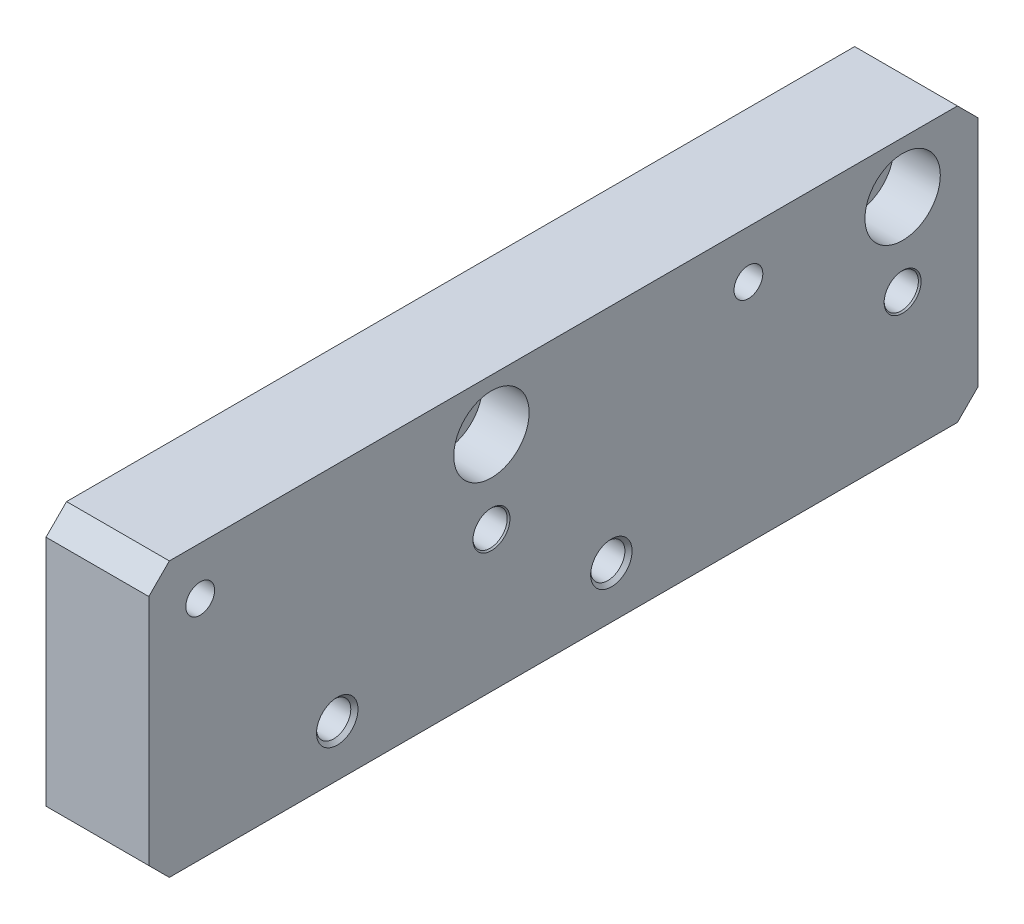
SolidWorks part; units mm, degrees
material "6061-T6"
ref_plane "Front Plane" through (0, 0, 0) normal (0, 0, 1) x (1, 0, 0)
ref_plane "Top Plane" through (0, 0, 0) normal (0, 1, 0) x (1, 0, 0)
ref_plane "Right Plane" through (0, 0, 0) normal (1, 0, 0) x (0, 0, -1)
sketch "Sketch1" plane through (0, 0, 0) normal (1, 0, 0) x (0, 0, -1)
  line L1 (-60.5, -20) -> (60.5, -20)
  line L2 (-60.5, -20) -> (-60.5, 20)
  line L3 (-60.5, 20) -> (60.5, 20)
  line L4 (60.5, -20) -> (60.5, 20)
  line L5 (-60.5, -20) -> (60.5, 20) construction
  line L6 (-60.5, 20) -> (60.5, -20) construction
  point P0 (0, 0)
  dimension "D1" = 40
  dimension "D2" = 121
extrude "Boss-Extrude1" add sketch "Sketch1" along normal blind 15
hole_wizard "M5 Tapped Hole1" positions "Sketch2" profile "Sketch3" tap size "M5" standard "GB"
sketch "Sketch2" plane through (15, 0, 0) normal (1, 0, 0) x (0, 0, -1)
  point P0 (-53, 13)
  point P3 (27, 13)
sketch "Sketch3" plane through (15, 13, 53) normal (0, 1, 0) x (0, 0, -1)
  line L0 (0, 0) -> (0, 13.6618)
  line L1 (0, 13.6618) -> (2.1, 12.4)
  line L2 (2.1, 12.4) -> (2.1, 0)
  line L5 (2.1, 0) -> (0, 0)
  line L10 (0, 13.6618) -> (-2.1, 12.4) construction
  line L11 (0, -6.35) -> (0, 107.95) construction
  dimension "螺纹孔钻头直径" = 4.2
  dimension "螺纹孔钻头深度" = 12.4
  dimension "导头角度" = 118
hole_wizard "M6 Tapped Hole1" positions "Sketch4" profile "Sketch5" tap size "M6" standard "GB"
sketch "Sketch4" plane through (15, 0, 0) normal (1, 0, 0) x (0, 0, -1)
  point P0 (-33, -12.5)
  point P3 (7, -12.5)
sketch "Sketch5" plane through (15, -12.5, 33) normal (0, 1, 0) x (0, 0, -1)
  line L0 (0, 0) -> (0, 16.5022)
  line L1 (0, 16.5022) -> (2.5, 15)
  line L2 (2.5, 15) -> (2.5, 0.525)
  line L3 (2.5, 0.525) -> (3.025, 0)
  line L5 (3.025, 0) -> (0, 0)
  line L6 (-2.5, 0.525) -> (-3.025, 0) construction
  line L10 (0, 16.5022) -> (-2.5, 15) construction
  line L11 (0, -6.35) -> (0, 107.95) construction
  dimension "螺纹孔钻头直径" = 5
  dimension "螺纹孔钻头深度" = 15
  dimension "近端锥形沉头孔直径" = 6.05
  dimension "近端锥形沉头孔角度" = 90
  dimension "导头角度" = 118
cosmetic thread "Cosmetic thread 1" parameters "D1"=12, "D2"=6
cosmetic thread "Cosmetic thread 2" parameters "D1"=12, "D2"=6
hole_wizard "CBORE for M6 Hexagon socket head cap screws1" positions "Sketch6" profile "Sketch7" counterbore size "M6" standard "GB" end condition through all
sketch "Sketch6" plane through (15, 0, 0) normal (1, 0, 0) x (0, 0, -1)
  line L1 (60.5, 20) -> (-60.5, 20) construction
  line L5 (-60.5, 20) -> (-60.5, -20) construction
  point P0 (-10.5, 12.5)
  point P2 (49.5, 12.5)
  dimension "D1" = 50
  dimension "D2" = 7.5
  dimension "D3" = 60
sketch "Sketch7" plane through (15, 12.5, 10.5) normal (0, 1, 0) x (0, 0, -1)
  line L0 (0, 0) -> (0, 15)
  line L1 (0, 15) -> (3.3, 15)
  line L3 (3.3, 15) -> (3.3, 6.8)
  line L4 (3.3, 6.8) -> (5.5, 6.8)
  line L5 (5.5, 6.8) -> (5.5, 0)
  line L7 (5.5, 0) -> (0, 0)
  line L11 (0, -6.35) -> (0, 107.95) construction
  dimension "通孔孔直径" = 6.6
  dimension "通孔孔深度" = 15
  dimension "柱形沉头孔直径" = 11
  dimension "柱形沉头孔深度" = 6.8
hole_wizard "Ø5.0mm blind hole 1" positions "Sketch8" profile "Sketch9" hole size "Ø5.0" standard "GB" end condition through all
sketch "Sketch8" plane through (15, 0, 0) normal (1, 0, 0) x (0, 0, -1)
  line L0 (49.5, 12.5) -> (49.5, 0.5) construction
  line L2 (-10.5, 12.5) -> (-10.5, 0.5) construction
  circle A0 centre (-10.5, 12.5) radius 3.3 construction
  point P0 (-10.5, 0.5)
  point P2 (49.5, 0.5)
  dimension "D1" = 12
sketch "Sketch9" plane through (15, 0.5, 10.5) normal (0, 1, 0) x (0, 0, -1)
  line L0 (0, 0) -> (0, 15)
  line L1 (0, 15) -> (2.5, 15)
  line L2 (2.5, 15) -> (2.5, 0.2)
  line L3 (2.5, 0.2) -> (2.7, 0)
  line L5 (2.7, 0) -> (0, 0)
  line L6 (-2.5, 0.2) -> (-2.7, 0) construction
  line L11 (0, -6.35) -> (0, 107.95) construction
  dimension "通孔孔直径" = 5
  dimension "通孔孔深度" = 15
  dimension "近端锥形沉头孔直径" = 5.4
  dimension "近端锥形沉头孔角度" = 90
chamfer "Chamfer1" distance 3 angle 45 4 edges at (7.5, 20, -60.5) (7.5, -20, -60.5) (7.5, 20, 60.5) (7.5, -20, 60.5)
